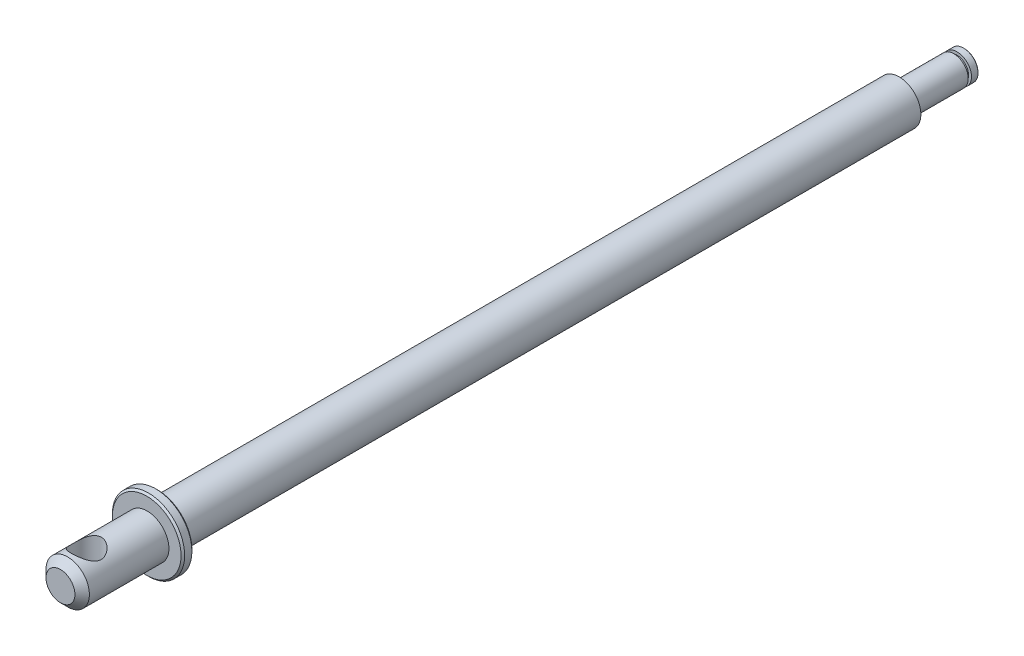
from build123d import *

# Parameters (mm, degrees)
SKETCH4_R          = 4
CUT_EXTRUDE2_DEPTH = 25
CHAMFER2_SIZE      = 2
CHAMFER3_SIZE      = 0.2
SKETCH5_R          = 10
BOSS_EXTRU_1_DEPTH = 3
CHAMFER4_SIZE      = 0.5


with BuildPart() as part:
    # Sketch1 → Revolve1 (revolve)
    with BuildSketch(Plane(origin=(0, 0, 0), x_dir=(1, 0, 0), z_dir=(0, 1, 0)), mode=Mode.PRIVATE) as revolve1_sk:
        Polygon((4.142447891, -208.268648203), (3.342447891, -208.268648203), (3.342447891, -209.168648203), (4.142447891, -209.168648203), (4.142447891, -224.268648203), (6.142447891, -224.268648203), (6.142447891, -456.268648203), (0.142447891, -456.268648203), (0.142447891, -206.268648203), (4.142447891, -206.268648203), align=None)
    revolve(revolve1_sk.sketch.rotate(Axis((0.142447891, 0, 206.268648203), (0, 0, 1)), 180), axis=Axis((0.142447891, 0, 206.268648203), (0, 0, 1)))

    # Sketch4 → Cut-Extrude2 (cut, symmetric)
    with BuildSketch(Plane(origin=(0, 0, 0), x_dir=(1, 0, 0), z_dir=(0, 1, 0))):
        with Locations(Location((0, -448.894244445, 0), (0, 0, 270))):
            Circle(SKETCH4_R)
    extrude(amount=CUT_EXTRUDE2_DEPTH, both=True, mode=Mode.SUBTRACT)

    # Chamfer2
    chamfer2_edges = [part.edges().sort_by_distance(p)[0] for p in [
        (6.142447891, 0, 456.268648203),
    ]]
    chamfer(chamfer2_edges, length=CHAMFER2_SIZE)

    # Chamfer3
    chamfer3_edges = [part.edges().sort_by_distance(p)[0] for p in [
        (4.142447891, 0, 206.268648203),
    ]]
    chamfer(chamfer3_edges, length=CHAMFER3_SIZE)

    # Sketch5 → Boss.-Extru.1 (add)
    with BuildSketch(Plane.XY.offset(429.268648203)):
        Circle(SKETCH5_R)
    extrude(amount=BOSS_EXTRU_1_DEPTH)

    # Chamfer4
    chamfer4_edges = [part.edges().sort_by_distance(p)[0] for p in [
        (-10, 0, 429.268648203),
        (-10, 0, 432.268648203),
    ]]
    chamfer(chamfer4_edges, length=CHAMFER4_SIZE)


solid = part.part
